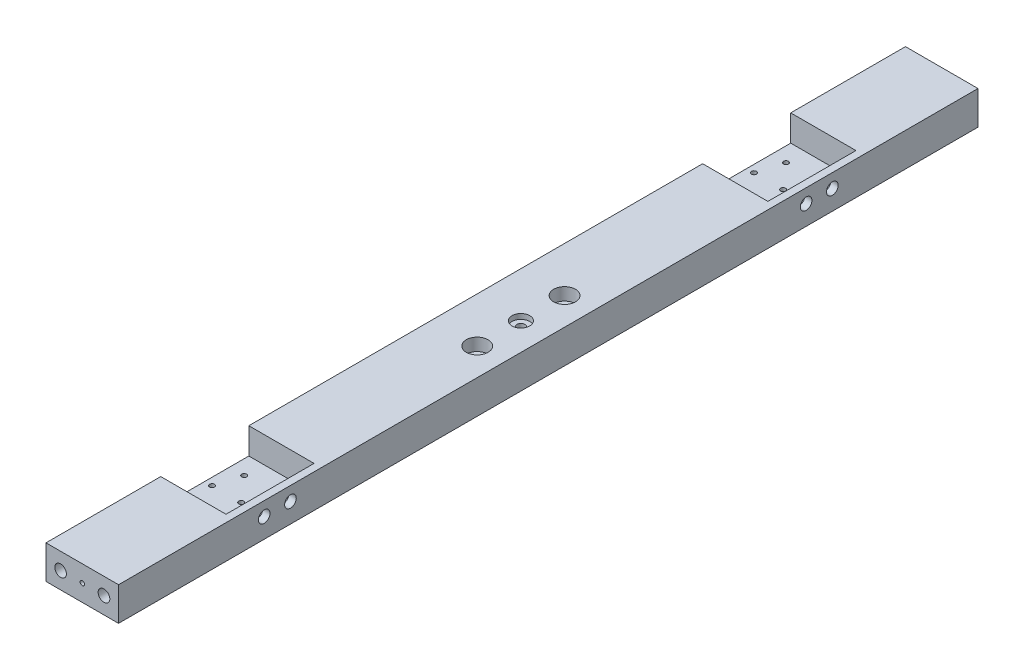
SolidWorks part; units mm, degrees
ref_plane "Front Plane" through (0, 0, 0) normal (0, 0, 1) x (1, 0, 0)
ref_plane "Top Plane" through (0, 0, 0) normal (0, 1, 0) x (1, 0, 0)
ref_plane "Right Plane" through (0, 0, 0) normal (1, 0, 0) x (0, 0, -1)
sketch "Sketch1" plane through (0, 0, 0) normal (0, 1, 0) x (1, 0, 0)
  line L1 (9, 295) -> (-31, 295)
  line L2 (9, 295) -> (9, -295)
  line L3 (9, -295) -> (-31, -295)
  line L4 (-31, 295) -> (-31, -295)
  point P0 (0, 0)
  point P6 (0, 0)
  dimension "D1" = 590
  dimension "D2" = 40
extrude "Boss-Extrude1" add sketch "Sketch1" along normal blind 23
sketch "Sketch2" plane through (-31, 0, 0) normal (-1, 0, 0) x (0, 0, 1)
  circle A0 centre (-270, 7.5) radius 2.25
  circle A1 centre (0, 7.5) radius 2.25
  circle A2 centre (270, 7.5) radius 2.25
sketch "Sketch4" plane through (0, 0, 295) normal (0, 0, 1) x (1, 0, 0)
  line L0 (9, 23) -> (-31, 0) construction
  circle A0 centre (-11, 11.5) radius 4.5374
sketch "Sketch6" plane through (0, 23, 0) normal (0, 1, 0) x (1, 0, 0)
  line L0 (-31, 0) -> (9, 0) construction
  line L1 (-31, 295) -> (-31, -295) construction
  line L2 (9, -295) -> (9, 295) construction
  circle A2 centre (0, -30) radius 2.5
  circle A3 centre (0, 30) radius 2.5
  circle A4 centre (0, 0) radius 2.2838
  dimension "D1" = 30
hole_wizard "CBORE for M8 Hex Socket Head Cap Screw0" positions "3DSketch4" profile "Sketch8" counterbore size "M8" standard "ISO"
sketch3d "3DSketch4"
  point P0 (0, 23, 30)
  point P6 (0, 23, -30)
sketch "Sketch8" plane through (0, 23, 30) normal (1, 0, 0) x (0, 0, 1)
  line L0 (0, 0) -> (0, 44.6439)
  line L1 (0, 44.6439) -> (4.5, 41.94)
  line L2 (4.5, 41.94) -> (4.5, 8.6)
  line L3 (4.5, 8.6) -> (7.5, 8.6)
  line L4 (7.5, 8.6) -> (7.5, 0)
  line L5 (7.5, 0) -> (0, 0)
  line L10 (0, 44.6439) -> (-4.5, 41.94) construction
  line L11 (0, -6.35) -> (0, 107.95) construction
  dimension "Hole Dia." = 9
  dimension "Hole Depth" = 41.94
  dimension "C'Bore Dia." = 15
  dimension "C'Bore Depth" = 8.6
  dimension "Drill Angle" = 118
sketch "Sketch9" plane through (0, 23, 0) normal (0, 1, 0) x (1, 0, 0)
  line L1 (-88.6463, -155.7724) -> (36.6463, -155.7724)
  line L2 (-88.6463, -155.7724) -> (-88.6463, -216.2276)
  line L3 (-88.6463, -216.2276) -> (36.6463, -216.2276)
  line L4 (36.6463, -155.7724) -> (36.6463, -216.2276)
  line L5 (-88.6463, -155.7724) -> (36.6463, -216.2276) construction
  line L6 (-88.6463, -216.2276) -> (36.6463, -155.7724) construction
  point P0 (-26, -186)
extrude "Cut-Extrude1" cut sketch "Sketch9" against normal blind 18
mirror "Mirror1" about plane through (0, 0, 0) normal (0, 0, 1) of "Cut-Extrude1"
sketch "Sketch11" plane through (0, 23, 0) normal (0, 1, 0) x (1, 0, 0)
  line L0 (9, -216.2276) -> (13.8, -216.2276)
  line L1 (9, 295) -> (13.8, 295)
  line L2 (9, 295) -> (9, 216.2276)
  line L3 (9, -295) -> (13.8, -295)
  line L4 (13.8, 295) -> (13.8, 216.2276)
  line L5 (9, -155.7724) -> (13.8, -155.7724)
  line L6 (9, 216.2276) -> (13.8, 216.2276)
  line L7 (9, 155.7724) -> (13.8, 155.7724)
  line L8 (9, -216.2276) -> (9, -295)
  line L9 (13.8, -216.2276) -> (13.8, -295)
  line L10 (13.8, 155.7724) -> (13.8, -155.7724)
  line L11 (9, 155.7724) -> (9, -155.7724)
extrude "Boss-Extrude2" add sketch "Sketch11" against normal up to surface (23 mm away) up to face at (0, 0, 25.5)
sketch "Sketch12" plane through (9, 0, 0) normal (1, 0, 0) x (0, 0, -1)
  line L4 (-216.2276, 0) -> (-155.7724, 0)
  line L5 (-155.7724, 0) -> (-155.7724, 5)
  line L6 (-155.7724, 5) -> (-216.2276, 5)
  line L7 (-216.2276, 5) -> (-216.2276, 0)
  line L8 (-216.2276, 0) -> (-155.7724, 0)
  line L9 (-155.7724, 0) -> (-155.7724, 5)
  line L10 (-155.7724, 5) -> (-216.2276, 5)
  line L11 (-216.2276, 5) -> (-216.2276, 0)
  dimension "D1" = 0
extrude "Boss-Extrude3" add sketch "Sketch12" along normal up to surface (4.8 mm away) up to face at (13.8, 11.5, 0)
mirror "Mirror2" about plane through (0, 0, 0) normal (0, 0, 1) of "Boss-Extrude3"
sketch "Sketch13" plane through (0, 23, 0) normal (0, 1, 0) x (1, 0, 0)
  line L0 (13.8, 295) -> (-31, 295) construction
  line L1 (13.8, -295) -> (18.8, -295)
  line L2 (13.8, -295) -> (13.8, 295)
  line L3 (13.8, 295) -> (18.8, 295)
  line L4 (18.8, -295) -> (18.8, 295)
  dimension "D1" = 5
extrude "Boss-Extrude4" add sketch "Sketch13" against normal up to surface (23 mm away) up to face at (0, 0, 25.5)
sketch "Sketch14" plane through (18.8, 0, 0) normal (1, 0, 0) x (0, 0, -1)
  circle A0 centre (-195, 13.5) radius 4
  circle A1 centre (-177, 13.5) radius 4
  dimension "D1" = 8
extrude "Cut-Extrude2" cut sketch "Sketch14" against normal blind 15
mirror "Mirror3" about plane through (0, 0, 0) normal (0, 0, 1) of "Cut-Extrude2"
sketch "Sketch15" plane through (0, 5, 0) normal (0, 1, 0) x (1, 0, 0)
  circle A0 centre (-21, -169) radius 1.7
  circle A1 centre (-6, -186) radius 1.7
  circle A2 centre (-26, -186) radius 1.7
  circle A3 centre (-21, -203) radius 1.7
extrude "Cut-Extrude3" cut sketch "Sketch15" against normal blind 15
mirror "Mirror4" about plane through (0, 0, 0) normal (0, 0, 1) of "Cut-Extrude3"
sketch "Sketch18" plane through (0, 23, 0) normal (0, 1, 0) x (1, 0, 0)
  point P0 (0, 0)
hole_wizard "CBORE for M5 Hex Head Bolt1" positions "3DSketch10" profile "Sketch20" counterbore size "M5" standard "ISO"
sketch3d "3DSketch10"
  point P0 (0, 23, 0)
sketch "Sketch20" plane through (0, 23, 0) normal (1, 0, 0) x (0, 0, 1)
  line L0 (0, 0) -> (0, 43.5924)
  line L1 (0, 43.5924) -> (2.75, 41.94)
  line L2 (2.75, 41.94) -> (2.75, 3.5)
  line L3 (2.75, 3.5) -> (6.119, 3.5)
  line L4 (6.119, 3.5) -> (6.119, 0)
  line L5 (6.119, 0) -> (0, 0)
  line L10 (0, 43.5924) -> (-2.75, 41.94) construction
  line L11 (0, -6.35) -> (0, 107.95) construction
  dimension "Hole Dia." = 5.5
  dimension "Hole Depth" = 41.94
  dimension "C'Bore Dia." = 12.238
  dimension "C'Bore Depth" = 3.5
  dimension "Drill Angle" = 118
sketch "Sketch21" plane through (0, 0, 295) normal (0, 0, 1) x (1, 0, 0)
  circle A0 centre (-21, 11.5) radius 5.6132
  circle A1 centre (8.8, 11.5) radius 4.5
  circle A2 centre (-6.1, 11.5) radius 4.016
hole_wizard "Ø8.0mm Dowel Hole1" positions "3DSketch11" profile "Sketch23" hole size "Ø8.0" standard "ISO"
sketch3d "3DSketch11"
  point P0 (-21, 11.5, 295)
  point P3 (8.8, 11.5, 295)
sketch "Sketch23" plane through (-21, 11.5, 295) normal (1, 0, 0) x (0, -1, 0)
  line L0 (0, 0) -> (0, 44.3434)
  line L1 (0, 44.3434) -> (4, 41.94)
  line L2 (4, 41.94) -> (4, 0)
  line L5 (4, 0) -> (0, 0)
  line L10 (0, 44.3434) -> (-4, 41.94) construction
  line L11 (0, -6.35) -> (0, 107.95) construction
  dimension "Hole Dia." = 8
  dimension "Hole Depth" = 41.94
  dimension "Drill Angle" = 118
hole_wizard "Ø3.0mm Dowel Hole1" positions "3DSketch12" profile "Sketch24" hole size "Ø3.0" standard "ISO"
sketch3d "3DSketch12"
  point P0 (-6.1, 11.5, 295)
sketch "Sketch24" plane through (-6.1, 11.5, 295) normal (1, 0, 0) x (0, -1, 0)
  line L0 (0, 0) -> (0, 42.8413)
  line L1 (0, 42.8413) -> (1.5, 41.94)
  line L2 (1.5, 41.94) -> (1.5, 0)
  line L5 (1.5, 0) -> (0, 0)
  line L10 (0, 42.8413) -> (-1.5, 41.94) construction
  line L11 (0, -6.35) -> (0, 107.95) construction
  dimension "Hole Dia." = 3
  dimension "Hole Depth" = 41.94
  dimension "Drill Angle" = 118
